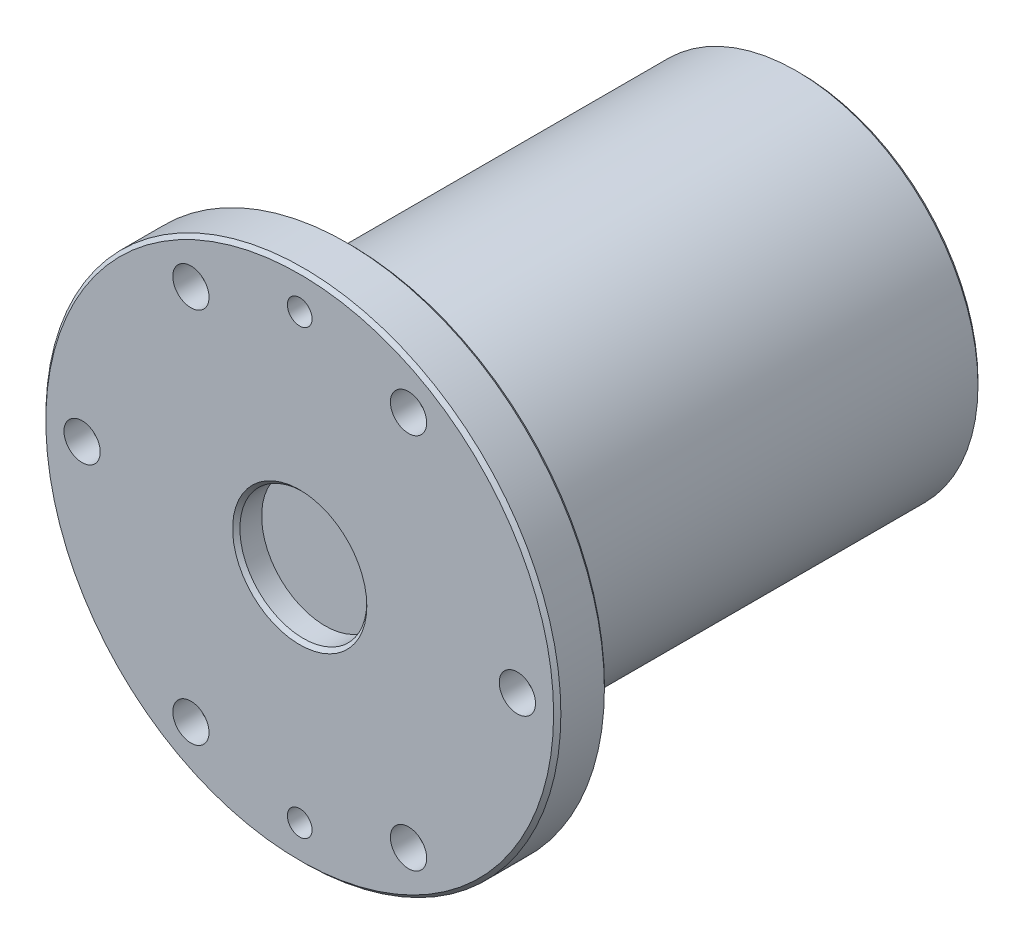
SolidWorks part; units mm, degrees
material "Cr12MoV"
ref_plane "Front Plane" through (0, 0, 0) normal (0, 0, 1) x (1, 0, 0)
ref_plane "Top Plane" through (0, 0, 0) normal (0, 1, 0) x (1, 0, 0)
ref_plane "Right Plane" through (0, 0, 0) normal (1, 0, 0) x (0, 0, -1)
sketch "Sketch1" plane through (0, 0, 0) normal (0, 0, 1) x (1, 0, 0)
  circle A0 centre (0, 0) radius 50
  dimension "D1" = 100
extrude "Boss-Extrude1" add sketch "Sketch1" along normal blind 138
sketch "Sketch6" plane through (0, 0, 138) normal (0, 0, 1) x (1, 0, 0)
  circle A0 centre (0, 0) radius 50
  circle A1 centre (0, 0) radius 71
  circle A2 centre (0, 0) radius 50 construction
  dimension "D1" = 142
extrude "Boss-Extrude2" add sketch "Sketch6" against normal blind 14
chamfer "Chamfer3" distance 1 angle 45 1 edges at (50, 0, 0)
chamfer "Chamfer4" distance 1 angle 45 1 edges at (71, 0, 138)
chamfer "Chamfer5" distance 1 angle 45 1 edges at (71, 0, 124)
sketch "Sketch7" plane through (0, 0, 138) normal (0, 0, 1) x (1, 0, 0)
  circle A0 centre (0, 0) radius 17.5
  dimension "D1" = 35
extrude "Cut-Extrude1" cut sketch "Sketch7" against normal blind 7
chamfer "Chamfer6" distance 1 angle 45 1 edges at (17.5, 0, 138)
hole_wizard "Hole size (per socket head cap screw type)1" positions "Sketch8" profile "Sketch9" counterbore size "M5" standard "GB"
sketch "Sketch8" plane through (0, 0, 138) normal (0, 0, 1) x (1, 0, 0)
  line L0 (-107.402, 0) -> (60, 0)
  circle A0 centre (0, 0) radius 60
  point P0 (60, 0)
  dimension "D1" = 120
sketch "Sketch9" plane through (60, 0, 138) normal (1, 0, 0) x (0, -1, 0)
  line L0 (0, 0) -> (0, 15.6524)
  line L1 (0, 15.6524) -> (2.75, 14)
  line L2 (2.75, 14) -> (2.75, 7)
  line L3 (2.75, 7) -> (5, 7)
  line L4 (5, 7) -> (5, 0)
  line L5 (5, 0) -> (0, 0)
  line L10 (0, 15.6524) -> (-2.75, 14) construction
  line L11 (0, -6.35) -> (0, 107.95) construction
  dimension "孔直径" = 5.5
  dimension "孔深度" = 14
  dimension "柱形沉头孔直径" = 10
  dimension "柱形沉头孔深度" = 7
  dimension "导头角度" = 118
pattern_circular "CirPattern1" count 6 over 360 about axis through (0, 0, 0) along (0, 0, 1) of "Hole size (per socket head cap screw type)1"
hole_wizard "M8 Tapped Hole1" positions "Sketch10" profile "Sketch11" tap size "M8" standard "GB" end condition through all
sketch "Sketch10" plane through (0, 0, 138) normal (0, 0, 1) x (1, 0, 0)
  line L0 (0, 0) -> (0, 61)
  circle A0 centre (0, 0) radius 61
  point P0 (0, 61)
  point P2 (0, -61)
  dimension "D1" = 122
sketch "Sketch11" plane through (0, 61, 138) normal (1, 0, 0) x (0, -1, 0)
  line L0 (0, 0) -> (0, 138)
  line L1 (0, 138) -> (3.4, 138)
  line L2 (3.4, 138) -> (3.4, 0)
  line L5 (3.4, 0) -> (0, 0)
  line L11 (0, -6.35) -> (0, 107.95) construction
  dimension "通孔螺纹孔钻头直径" = 6.8
  dimension "通孔螺纹孔钻头深度" = 138
cosmetic thread "Cosmetic thread 1" parameters "D2"=8
cosmetic thread "Cosmetic thread 2" parameters "D2"=8
